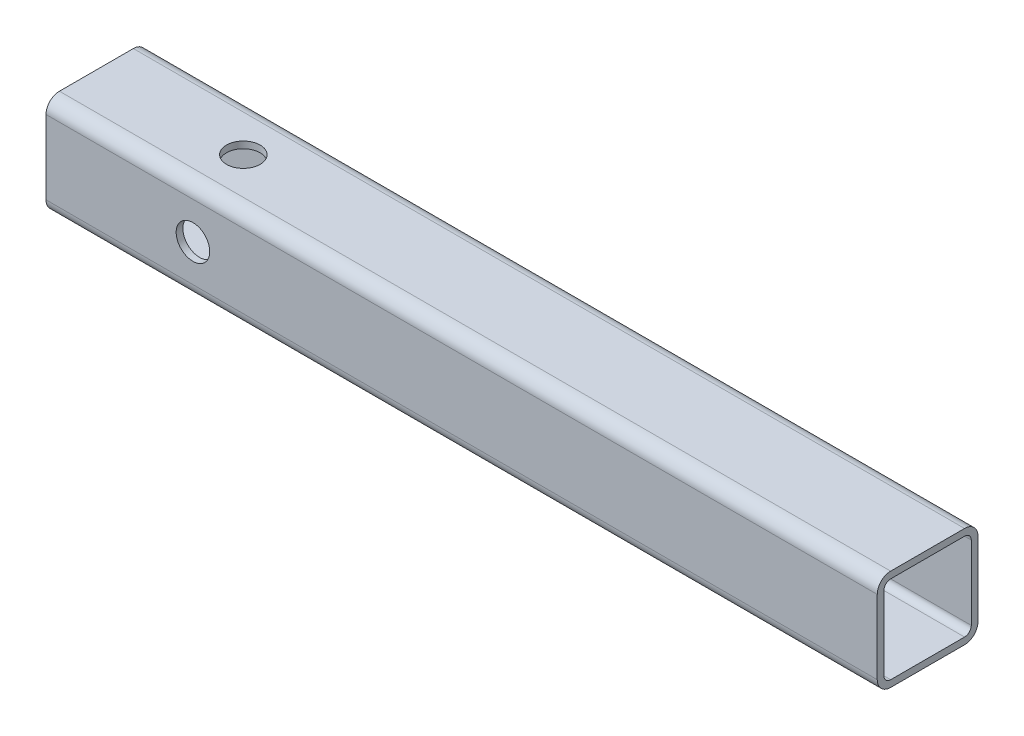
SolidWorks part; units mm, degrees
material "普通碳钢"
ref_plane "前视基准面" through (0, 0, 0) normal (0, 0, 1) x (1, 0, 0)
ref_plane "上视基准面" through (0, 0, 0) normal (0, 1, 0) x (1, 0, 0)
ref_plane "右视基准面" through (0, 0, 0) normal (1, 0, 0) x (0, 0, -1)
sketch "草图1" plane through (0, 0, 0) normal (0, 0, 1) x (1, 0, 0)
  line L0 (-247.5, 0) -> (247.5, 0)
  point P4 (0, 0)
  dimension "D1" = 495
other "冷弯空心方管gb∕t6728-2002 60 X 60 X 4(1)"
ref_plane "基准面1" through (-247.5, 0, 0) normal (1, 0, 0) x (0, 1, 0)
sketch "Sketch1" plane through (-247.5, 0, 0) normal (1, 0, 0) x (0, 1, 0)
  line L0 (-22, -26) -> (22, -26)
  line L1 (-26, -22) -> (-26, 22)
  line L2 (22, 26) -> (-22, 26)
  line L3 (26, 22) -> (26, -22)
  line L4 (-22, -30) -> (22, -30)
  line L5 (-30, -22) -> (-30, 22)
  line L6 (22, 30) -> (-22, 30)
  line L7 (30, 22) -> (30, -22)
  arc A0 (30, 22) -> (22, 30) centre (22, 22) ccw
  arc A1 (22, -30) -> (30, -22) centre (22, -22) ccw
  arc A2 (-30, -22) -> (-22, -30) centre (-22, -22) ccw
  arc A3 (-22, 30) -> (-30, 22) centre (-22, 22) ccw
  arc A4 (-22, 26) -> (-26, 22) centre (-22, 22) ccw
  arc A5 (26, 22) -> (22, 26) centre (22, 22) ccw
  arc A6 (22, -26) -> (26, -22) centre (22, -22) ccw
  arc A7 (-26, -22) -> (-22, -26) centre (-22, -22) ccw
  point P0 (-30, 0)
  point P1 (30, 0)
  point P2 (0, 30)
  point P3 (0, -30)
  point P4 (0, 0)
  point P5 (-30, -30)
  point P6 (30, -30)
  point P7 (30, 30)
  point P8 (-30, 30)
  point P33 (0, 0)
  dimension "D1" = 8
  dimension "Thickness" = 4
  dimension "V_leg" = 60
sketch "草图5" plane through (0, 0, 30) normal (0, 0, 1) x (1, 0, 0)
  circle A0 centre (-160, 0) radius 10
  dimension "D1" = 20
  dimension "D2" = 160
extrude "切除-拉伸1" cut sketch "草图5" against normal up to surface (60 mm away) up to face at (0, 0, -30)
sketch "草图6" plane through (0, 30, 0) normal (0, 1, 0) x (1, 0, 0)
  circle A0 centre (-160, 0) radius 10
  dimension "D1" = 20
  dimension "D2" = 160
extrude "切除-拉伸2" cut sketch "草图6" against normal up to surface (60 mm away) up to face at (0, -30, 0)
